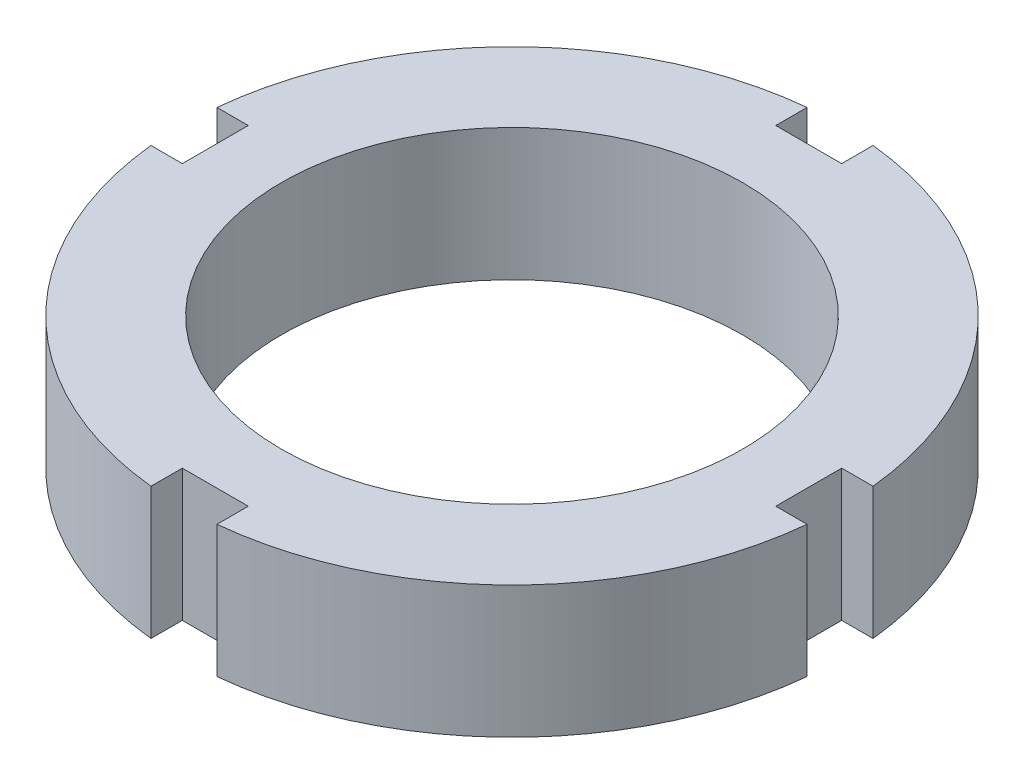
SolidWorks part; units mm, degrees
material "45"
ref_plane "Front Plane" through (0, 0, 0) normal (0, 0, 1) x (1, 0, 0)
ref_plane "Top Plane" through (0, 0, 0) normal (0, 1, 0) x (1, 0, 0)
ref_plane "Right Plane" through (0, 0, 0) normal (1, 0, 0) x (0, 0, -1)
sketch "Sketch1" plane through (0, 0, 0) normal (0, 1, 0) x (1, 0, 0)
  line L0 (0, 0) -> (0, 74.8513) construction
  line L1 (-5, 49.7494) -> (-5, 45)
  line L2 (-5, 45) -> (5, 45)
  line L3 (5, 45) -> (5, 49.7494)
  line L4 (45, 5) -> (45, -5)
  line L5 (49.7494, 5) -> (45, 5)
  line L6 (45, -5) -> (49.7494, -5)
  line L7 (5, -45) -> (-5, -45)
  line L8 (5, -49.7494) -> (5, -45)
  line L9 (-5, -45) -> (-5, -49.7494)
  line L10 (-45, -5) -> (-45, 5)
  line L11 (-49.7494, -5) -> (-45, -5)
  line L12 (-45, 5) -> (-49.7494, 5)
  arc A0 (-5, 49.7494) -> (-49.7494, 5) centre (0, 0) ccw
  circle A1 centre (0, 0) radius 35
  arc A2 (-49.7494, -5) -> (-5, -49.7494) centre (0, 0) ccw
  arc A3 (5, -49.7494) -> (49.7494, -5) centre (0, 0) ccw
  arc A4 (49.7494, 5) -> (5, 49.7494) centre (0, 0) ccw
  point P23 (0, 0)
  dimension "D1" = 100
  dimension "D2" = 70
  dimension "D3" = 10
  dimension "D4" = 45
  dimension "D5" = 4
extrude "Boss-Extrude1" add sketch "Sketch1" along normal blind 20
